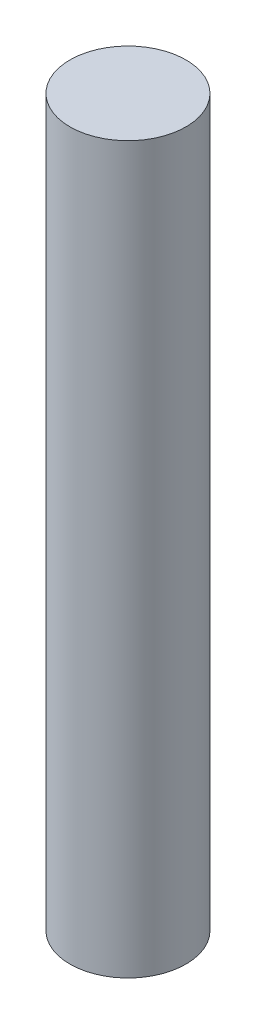
from build123d import *

# Parameters (mm, degrees)
SKETCH1_R           = 8
BOSS_EXTRUDE1_DEPTH = 100


with BuildPart() as part:
    # Sketch1 → Boss-Extrude1 (new body)
    with BuildSketch(Plane(origin=(0, 0, 0), x_dir=(1, 0, 0), z_dir=(0, 1, 0))):
        with Locations(Location((0, 0, 0), (0, 0, 270))):
            Circle(SKETCH1_R)
    extrude(amount=BOSS_EXTRUDE1_DEPTH)


solid = part.part
